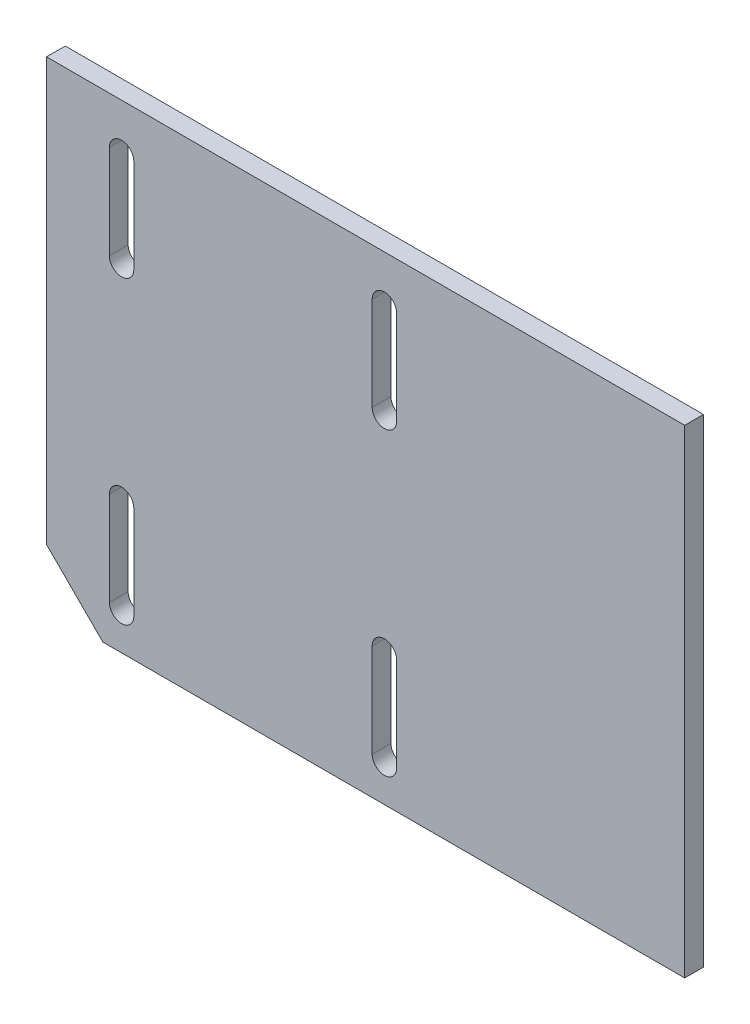
SolidWorks part; units mm, degrees
material "普通碳钢"
ref_plane "Front Plane" through (0, 0, 0) normal (0, 0, 1) x (1, 0, 0)
ref_plane "Top Plane" through (0, 0, 0) normal (0, 1, 0) x (1, 0, 0)
ref_plane "Right Plane" through (0, 0, 0) normal (1, 0, 0) x (0, 0, -1)
sketch "Sketch1" plane through (0, 0, 0) normal (0, 0, 1) x (1, 0, 0)
  line L0 (0, 0) -> (-340, 0)
  line L1 (-340, 0) -> (-340, -225)
  line L2 (-310, -255) -> (0, -255)
  line L3 (0, -255) -> (0, 0)
  line L4 (-340, -225) -> (-310, -255)
  line L5 (-300, -25) -> (-300, -75) construction
  line L6 (-293.5, -25) -> (-293.5, -75)
  line L7 (-306.5, -25) -> (-306.5, -75)
  line L8 (-160, -25) -> (-160, -75) construction
  line L9 (-153.5, -25) -> (-153.5, -75)
  line L10 (-166.5, -25) -> (-166.5, -75)
  line L11 (-300, -185) -> (-300, -235) construction
  line L12 (-293.5, -185) -> (-293.5, -235)
  line L13 (-306.5, -185) -> (-306.5, -235)
  line L14 (-160, -185) -> (-160, -235) construction
  line L15 (-153.5, -185) -> (-153.5, -235)
  line L16 (-166.5, -185) -> (-166.5, -235)
  arc A0 (-293.5, -25) -> (-306.5, -25) centre (-300, -25) ccw
  arc A1 (-306.5, -75) -> (-293.5, -75) centre (-300, -75) ccw
  arc A2 (-153.5, -25) -> (-166.5, -25) centre (-160, -25) ccw
  arc A3 (-166.5, -75) -> (-153.5, -75) centre (-160, -75) ccw
  arc A4 (-293.5, -185) -> (-306.5, -185) centre (-300, -185) ccw
  arc A5 (-306.5, -235) -> (-293.5, -235) centre (-300, -235) ccw
  arc A6 (-153.5, -185) -> (-166.5, -185) centre (-160, -185) ccw
  arc A7 (-166.5, -235) -> (-153.5, -235) centre (-160, -235) ccw
  point P4 (-340, -255)
  point P9 (-300, -50)
  point P14 (-160, -50)
  point P21 (-300, -210)
  point P28 (-160, -210)
  dimension "D1" = 340
  dimension "D2" = 255
  dimension "D3" = 140
  dimension "D4" = 40
  dimension "D6" = 160
  dimension "D7" = 50
  dimension "D8" = 50
  dimension "D9" = 13
extrude "Boss-Extrude1" add sketch "Sketch1" against normal blind 10
